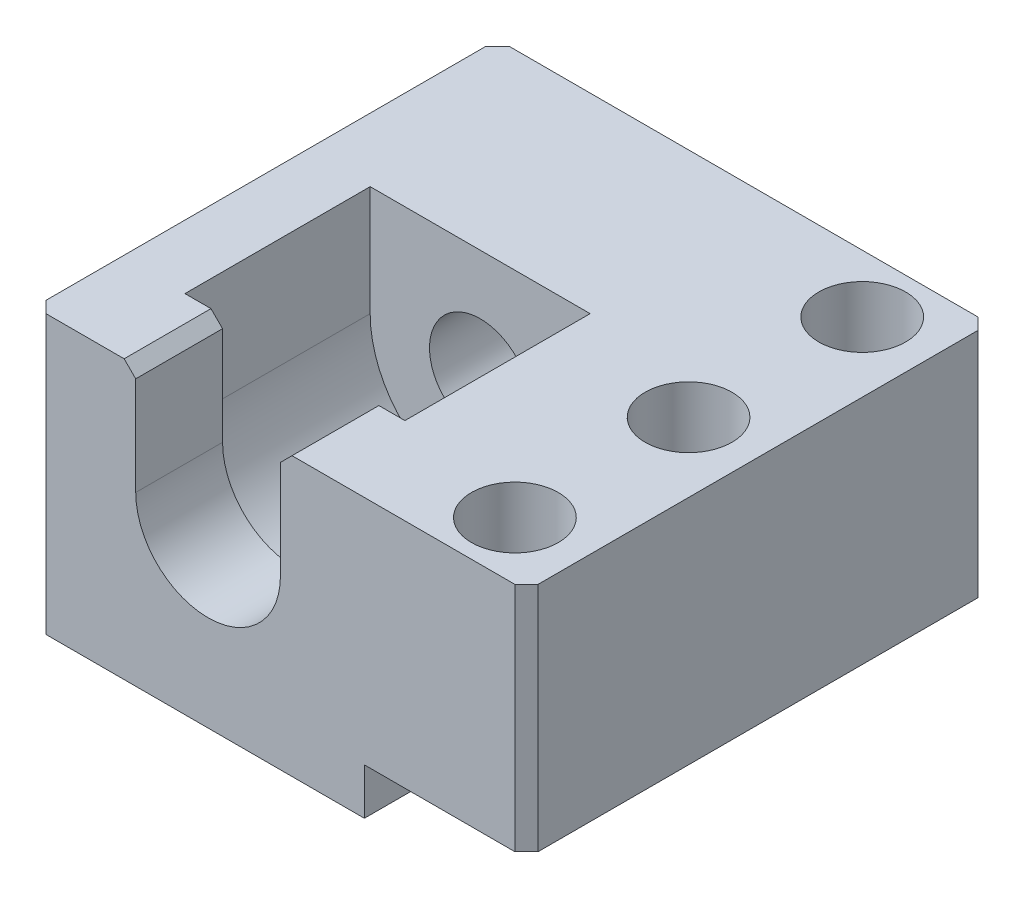
from build123d import *

# Parameters (mm, degrees)
BOSS_EXTRUDE1_DEPTH = 80
CUT_EXTRUDE1_DEPTH  = 15
CUT_EXTRUDE2_DEPTH  = 32
M20_TAPPED_HOLE1_D  = 17.5
HOLE1_D             = 8.4
HOLE1_CBORE_D       = 15
HOLE1_CBORE_DEPTH   = 20
CHAMFER1_SIZE       = 2


with BuildPart() as part:
    # Sketch2 → Boss-Extrude1 (new body)
    with BuildSketch(Plane.XY):
        Polygon((-36.962834249, 9.808501666), (-36.962834249, -38.191498334), (20.037165751, -38.191498334), (20.037165751, -30.191498334), (48.037165751, -30.191498334), (48.037165751, 9.808501666), align=None)
    extrude(amount=BOSS_EXTRUDE1_DEPTH)

    # Sketch3 → Cut-Extrude1 (cut)
    with BuildSketch(Plane.XY.offset(80)):
        with BuildLine():
            Line((-19.462834249, -9.191498334), (-19.462834249, 9.808501666))
            Line((-19.462834249, 9.808501666), (5.537165751, 9.808501666))
            Line((5.537165751, 9.808501666), (5.537165751, -9.191498334))
            ThreePointArc((5.537165751, -9.191498334), (-6.962834249, -21.691498334), (-19.462834249, -9.191498334))
        make_face()
    extrude(amount=-CUT_EXTRUDE1_DEPTH, mode=Mode.SUBTRACT)

    # Sketch4 → Cut-Extrude2 (cut)
    with BuildSketch(Plane.XY.offset(65)):
        with BuildLine():
            Line((-25.962834249, -9.191498334), (-25.962834249, 9.808501666))
            Line((-25.962834249, 9.808501666), (12.037165751, 9.808501666))
            Line((12.037165751, 9.808501666), (12.037165751, -9.191498334))
            ThreePointArc((12.037165751, -9.191498334), (-6.962834249, -28.191498334), (-25.962834249, -9.191498334))
        make_face()
    extrude(amount=-CUT_EXTRUDE2_DEPTH, mode=Mode.SUBTRACT)

    # M20 Tapped Hole1 (through all)
    with Locations(Plane.XY.offset(33)):
        with Locations((-6.962834249, -9.191498334)):
            Hole(M20_TAPPED_HOLE1_D / 2)

    # Hole1 (through all)
    with Locations(Plane(origin=(0, 9.808501666, 0), x_dir=(1, 0, 0), z_dir=(0, 1, 0))):
        with Locations((36.037165751, -10), (36.037165751, -40), (36.037165751, -70)):
            CounterBoreHole(HOLE1_D / 2, HOLE1_CBORE_D / 2, HOLE1_CBORE_DEPTH)

    # Chamfer1
    chamfer1_edges = [part.edges().sort_by_distance(p)[0] for p in [
        (-19.462834249, 9.808501666, 72.5),
        (48.037165751, -10.191498334, 80),
        (5.537165751, 9.808501666, 72.5),
        (48.037165751, -10.191498334, 0),
        (-36.962834249, -14.191498334, 0),
        (-36.962834249, -14.191498334, 80),
    ]]
    chamfer(chamfer1_edges, length=CHAMFER1_SIZE)


solid = part.part
